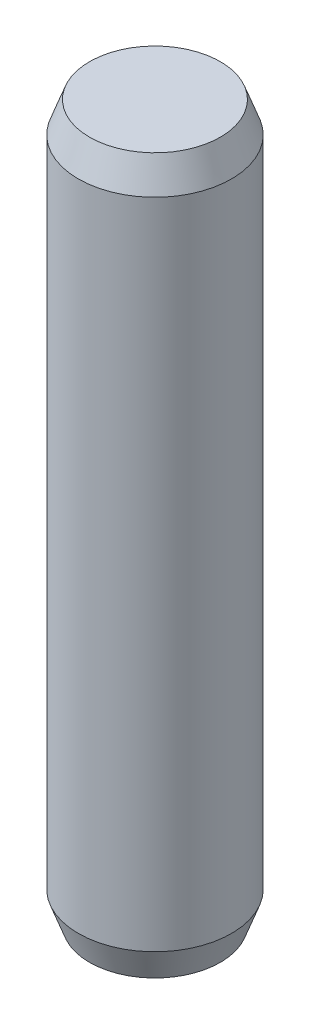
SolidWorks part; units mm, degrees
material "35"
ref_plane "Front Plane" through (0, 0, 0) normal (0, 0, 1) x (1, 0, 0)
ref_plane "Top Plane" through (0, 0, 0) normal (0, 1, 0) x (1, 0, 0)
ref_plane "Right Plane" through (0, 0, 0) normal (1, 0, 0) x (0, 0, -1)
sketch "Sketch1" plane through (0, 0, 0) normal (0, 1, 0) x (1, 0, 0)
  circle A0 centre (0, 0) radius 3
  dimension "D1" = 6
extrude "Boss-Extrude1" add sketch "Sketch1" along normal mid plane 28
chamfer "Chamfer1" distance 1.2 angle 20 1 edges at (0, 14, 3)
chamfer "Chamfer2" distance 1.2 angle 20 1 edges at (0, -14, 3)
